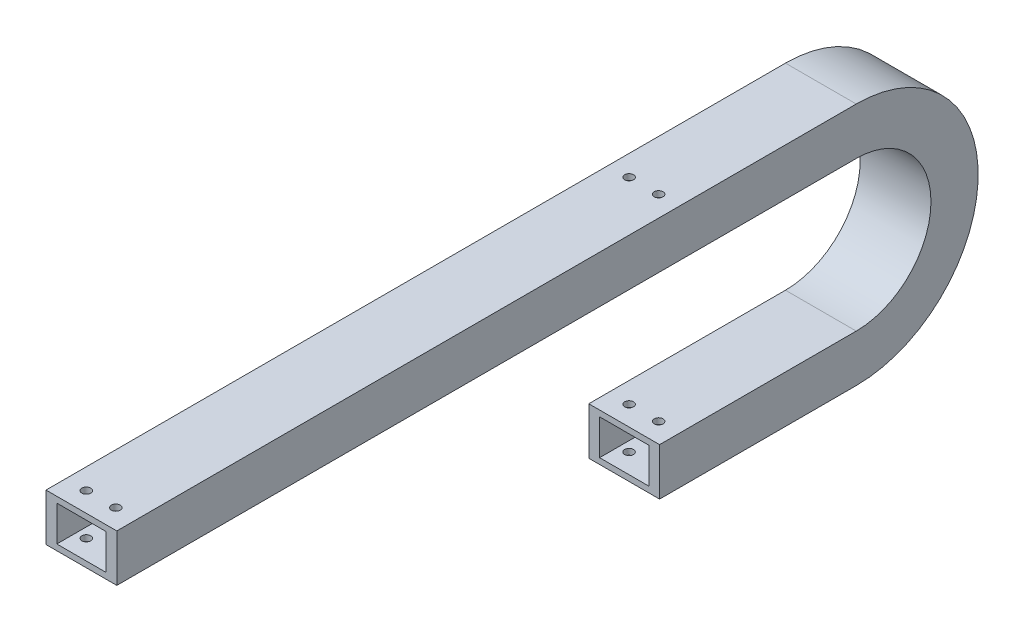
from build123d import *

# Parameters (mm, degrees)
SKETCH_2_W          = 36
SKETCH_2_H          = 24
SKETCH_2_W_2        = 25
SKETCH_2_H_2        = 18
SKETCH_4_R          = 2.25
CUT_EXTRUDE_1_DEPTH = 304.110540892


with BuildPart() as part:
    # 扫描1: sweep along a path in 草图3
    with BuildLine(Plane(origin=(0, 0, 0), x_dir=(0, 0, -1), z_dir=(1, 0, 0))) as sweep_1_path:
        Line((0, 0), (100, 0))
        ThreePointArc((100, 0), (150, 50), (100, 100))
        Line((100, 100), (-276, 100))
    # 草图2 → 扫描1 (sweep)
    with BuildSketch(Plane.XY):
        Rectangle(SKETCH_2_W, SKETCH_2_H)
        Rectangle(SKETCH_2_W_2, SKETCH_2_H_2, mode=Mode.SUBTRACT)
    sweep(path=sweep_1_path.line)

    # 草图4 → 切除-拉伸1 (cut, through all)
    with BuildSketch(Plane.XZ.offset(12)):
        with Locations(Location((-7.5, -10, 0), (0, 0, 180))):
            Circle(SKETCH_4_R)
        with Locations(Location((7.5, -10, 0), (0, 0, 180))):
            Circle(SKETCH_4_R)
        with Locations(Location((-7.5, 266, 0), (0, 0, 270))):
            Circle(SKETCH_4_R)
        with Locations(Location((7.5, 266, 0), (0, 0, 270))):
            Circle(SKETCH_4_R)
    extrude(amount=-CUT_EXTRUDE_1_DEPTH, mode=Mode.SUBTRACT)


solid = part.part
